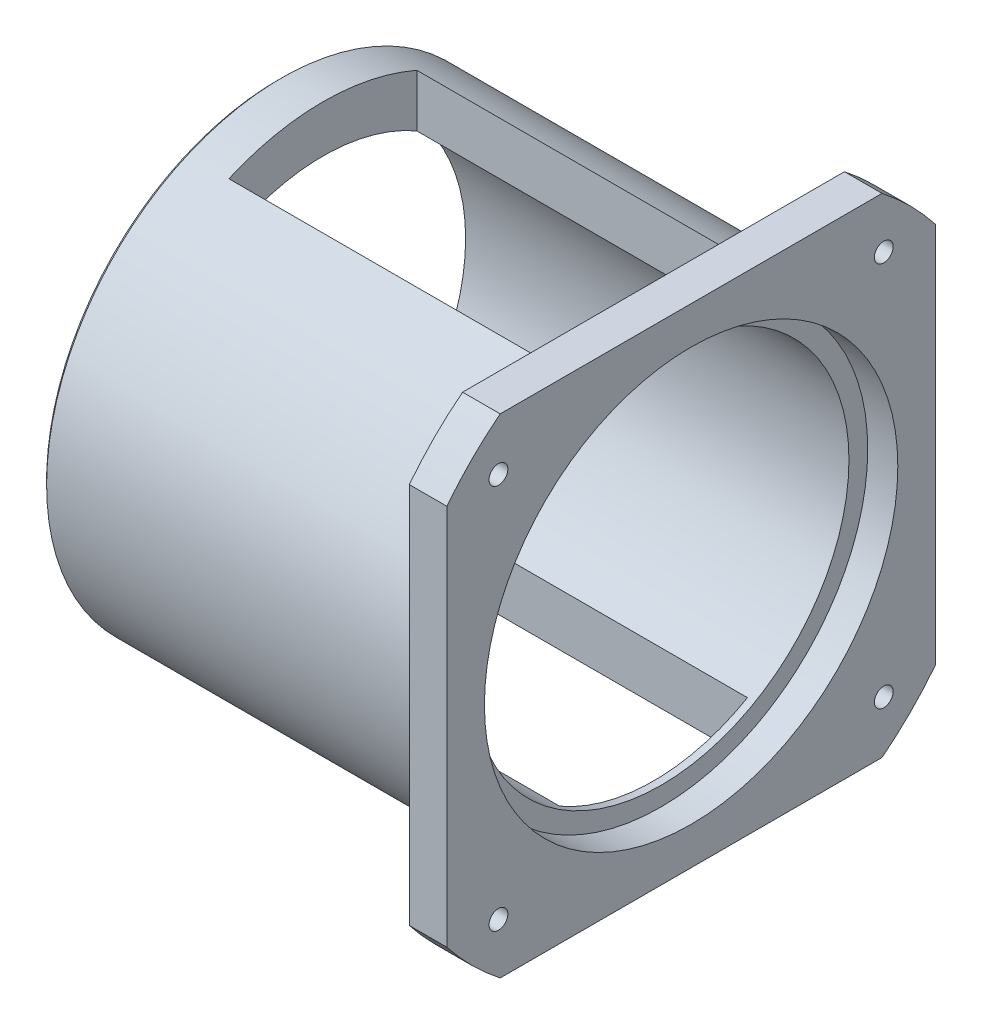
from build123d import *

# Parameters (mm, degrees)
SKETCH_1_R               = 62.5
EXTRUDE_1_DEPTH          = 100
SKETCH_2_R               = 82.5
EXTRUDE_2_DEPTH          = 10
SKETCH_3_OUTSIDE_W       = 218.594
SKETCH_3_OUTSIDE_H       = 218.594
SKETCH_3_OUTSIDE_W_2     = 130
SKETCH_3_OUTSIDE_H_2     = 130
CUT_EXTRUDE_1_DEPTH      = 161.351177108
SKETCH_4_R               = 55
CUT_EXTRUDE_2_DEPTH      = 8
PATTERN_CIRCULAR_1_COUNT = 4
SKETCH_7_R               = 50
CUT_EXTRUDE_3_DEPTH      = 138.309868546
CUT_EXTRUDE_4_DEPTH      = 144.352711868
CUT_EXTRUDE_4_DEPTH_BACK = 144.352711868
SKETCH_8_W               = 88
SKETCH_8_H               = 50
PATTERN_CIRCULAR_2_COUNT = 4
CHAMFER_1_SIZE           = 1


with BuildPart() as part:
    # 草图1 → 凸台-拉伸1 (new body)
    with BuildSketch(Plane(origin=(0, 0, 0), x_dir=(0, 0, -1), z_dir=(1, 0, 0))):
        Circle(SKETCH_1_R)
    extrude(amount=EXTRUDE_1_DEPTH)

    # 草图2 → 凸台-拉伸2 (add)
    with BuildSketch(Plane(origin=(100, 0, 0), x_dir=(0, 0, -1), z_dir=(1, 0, 0))):
        Circle(SKETCH_2_R)
    extrude(amount=EXTRUDE_2_DEPTH)

    # 草图3 outside → 切除-拉伸1 (cut, through all)
    with BuildSketch(Plane(origin=(110, 0, 0), x_dir=(0, 0, -1), z_dir=(1, 0, 0))):
        Rectangle(SKETCH_3_OUTSIDE_W, SKETCH_3_OUTSIDE_H)
        Rectangle(SKETCH_3_OUTSIDE_W_2, SKETCH_3_OUTSIDE_H_2, mode=Mode.SUBTRACT)
    extrude(amount=-CUT_EXTRUDE_1_DEPTH, mode=Mode.SUBTRACT)

    # 草图4 → 切除-拉伸2 (cut)
    with BuildSketch(Plane(origin=(110, 0, 0), x_dir=(0, 0, -1), z_dir=(1, 0, 0))):
        Circle(SKETCH_4_R)
    extrude(amount=-CUT_EXTRUDE_2_DEPTH, mode=Mode.SUBTRACT)

    # 草图6 → M6 螺纹孔1 (revolve, cut)
    with BuildSketch(Plane(origin=(110, 51.265241636, 51.265241636), x_dir=(0, 0, -1), z_dir=(0, 1, 0))):
        Polygon((0, 0), (0, 16.502151548), (2.5, 15), (2.5, 0), align=None)
    hole_wizard_m6_1 = revolve(axis=Axis((116.35, 51.265241636, 51.265241636), (-1, 0, 0)), mode=Mode.SUBTRACT)

    # 阵列(圆周)1: M6 螺纹孔1 ×4 about axis
    pattern_circular_1_axis = Axis((0, 0, 0), (1, 0, 0))
    for i in range(1, PATTERN_CIRCULAR_1_COUNT):
        add(hole_wizard_m6_1.rotate(pattern_circular_1_axis, i * 360 / PATTERN_CIRCULAR_1_COUNT), mode=Mode.SUBTRACT)

    # 草图7 → 切除-拉伸3 (cut, through all)
    with BuildSketch(Plane(origin=(102, 0, 0), x_dir=(0, 0, -1), z_dir=(1, 0, 0))):
        Circle(SKETCH_7_R)
    extrude(amount=-CUT_EXTRUDE_3_DEPTH, mode=Mode.SUBTRACT)

    # 草图8 → 切除-拉伸4 (cut, two sides: drawn at the far end of the back side and taken through both)
    with BuildSketch(Plane(origin=(0, 0, 0), x_dir=(1, 0, 0), z_dir=(0, 1, 0)).offset(-CUT_EXTRUDE_4_DEPTH_BACK)):
        with Locations((56, 0)):
            Rectangle(SKETCH_8_W, SKETCH_8_H)
    extrude(amount=CUT_EXTRUDE_4_DEPTH + CUT_EXTRUDE_4_DEPTH_BACK, mode=Mode.SUBTRACT)

    # 草图10 → M8 螺纹孔1 (revolve, cut)
    with BuildSketch(Plane(origin=(0, 39.597979746, -39.597979746), x_dir=(0, 0, 1), z_dir=(0, 1, 0))):
        Polygon((0, 0), (0, 21.792926105), (3.4, 19.75), (3.4, 0), align=None)
    hole_wizard_m8_1 = revolve(axis=Axis((-6.35, 39.597979746, -39.597979746), (1, 0, 0)), mode=Mode.SUBTRACT)

    # 阵列(圆周)2: M8 螺纹孔1 ×4 about axis
    pattern_circular_2_axis = Axis((0, 0, 0), (1, 0, 0))
    for i in range(1, PATTERN_CIRCULAR_2_COUNT):
        add(hole_wizard_m8_1.rotate(pattern_circular_2_axis, i * 360 / PATTERN_CIRCULAR_2_COUNT), mode=Mode.SUBTRACT)

    # 倒角1
    chamfer_1_edges = [part.edges().sort_by_distance(p)[0] for p in [
        (0, 0, 62.5),
    ]]
    chamfer(chamfer_1_edges, length=CHAMFER_1_SIZE)


solid = part.part
